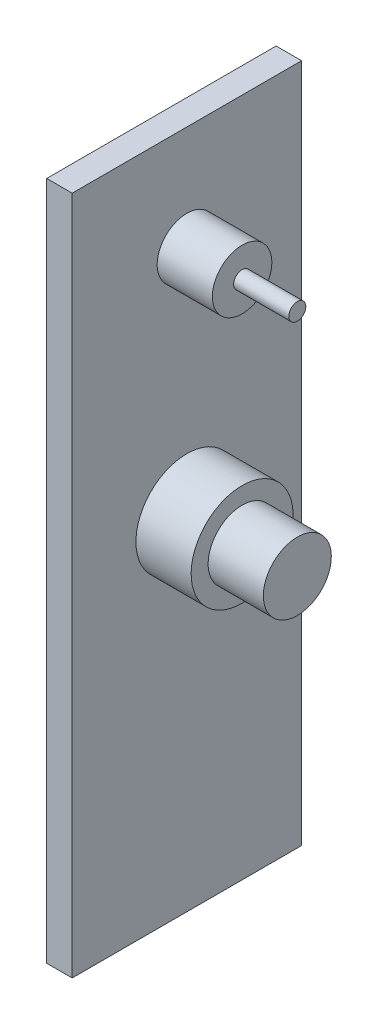
from build123d import *

# Parameters (mm, degrees)
SKETCH_1_W          = 3
SKETCH_1_H          = 80
EXTRUDE_1_DEPTH     = 27
SKETCH_2_R          = 3.5
SKETCH_2_R_2        = 6
EXTRUDE_2_DEPTH     = 6.5
SKETCH_3_R          = 1
SKETCH_3_R_2        = 4
EXTRUDE_3_DEPTH     = 6.5
SKETCH_4_R          = 1
CUT_EXTRUDE_1_DEPTH = 15


with BuildPart() as part:
    # 草图1 → 凸台-拉伸1 (new body)
    with BuildSketch(Plane.XY):
        with Locations((0.517241379, 39.071316614)):
            Rectangle(SKETCH_1_W, SKETCH_1_H)
    extrude(amount=EXTRUDE_1_DEPTH)

    # 草图2 → 凸台-拉伸2 (add)
    with BuildSketch(Plane(origin=(2.017241379, 0, 0), x_dir=(0, 0, -1), z_dir=(1, 0, 0))):
        with Locations(Location((-13.5, 66.771316614, 0), (0, 0, 270))):
            Circle(SKETCH_2_R)
        with Locations(Location((-13.5, 39.771316614, 0), (0, 0, 270))):
            Circle(SKETCH_2_R_2)
    extrude(amount=EXTRUDE_2_DEPTH)

    # 草图3 → 凸台-拉伸3 (add)
    with BuildSketch(Plane(origin=(8.517241379, 0, 0), x_dir=(0, 0, -1), z_dir=(1, 0, 0))):
        with Locations(Location((-13.5, 66.771316614, 0), (0, 0, 270))):
            Circle(SKETCH_3_R)
        with Locations(Location((-13.5, 39.771316614, 0), (0, 0, 270))):
            Circle(SKETCH_3_R_2)
    extrude(amount=EXTRUDE_3_DEPTH)

    # 草图4 → 切除-拉伸1 (cut)
    with BuildSketch(Plane(origin=(-1096.213929055, -10.928683386, 855.0606199), x_dir=(0.12186934340512692, -2.2319547324357124e-14, -0.9925461516413246), z_dir=(0, -1, 0))):
        with Locations((963.085867609, 999.8129825)):
            Circle(SKETCH_4_R)
        with Locations((977.974059883, 997.984942349)):
            Circle(SKETCH_4_R)
        with Locations(Location((961.501566145, 986.909882529, 0), (0, 0, 83))):
            Circle(SKETCH_4_R)
        with Locations(Location((976.389758419, 985.081842378, 0), (0, 0, 83))):
            Circle(SKETCH_4_R)
    extrude(amount=-CUT_EXTRUDE_1_DEPTH, mode=Mode.SUBTRACT)


solid = part.part
